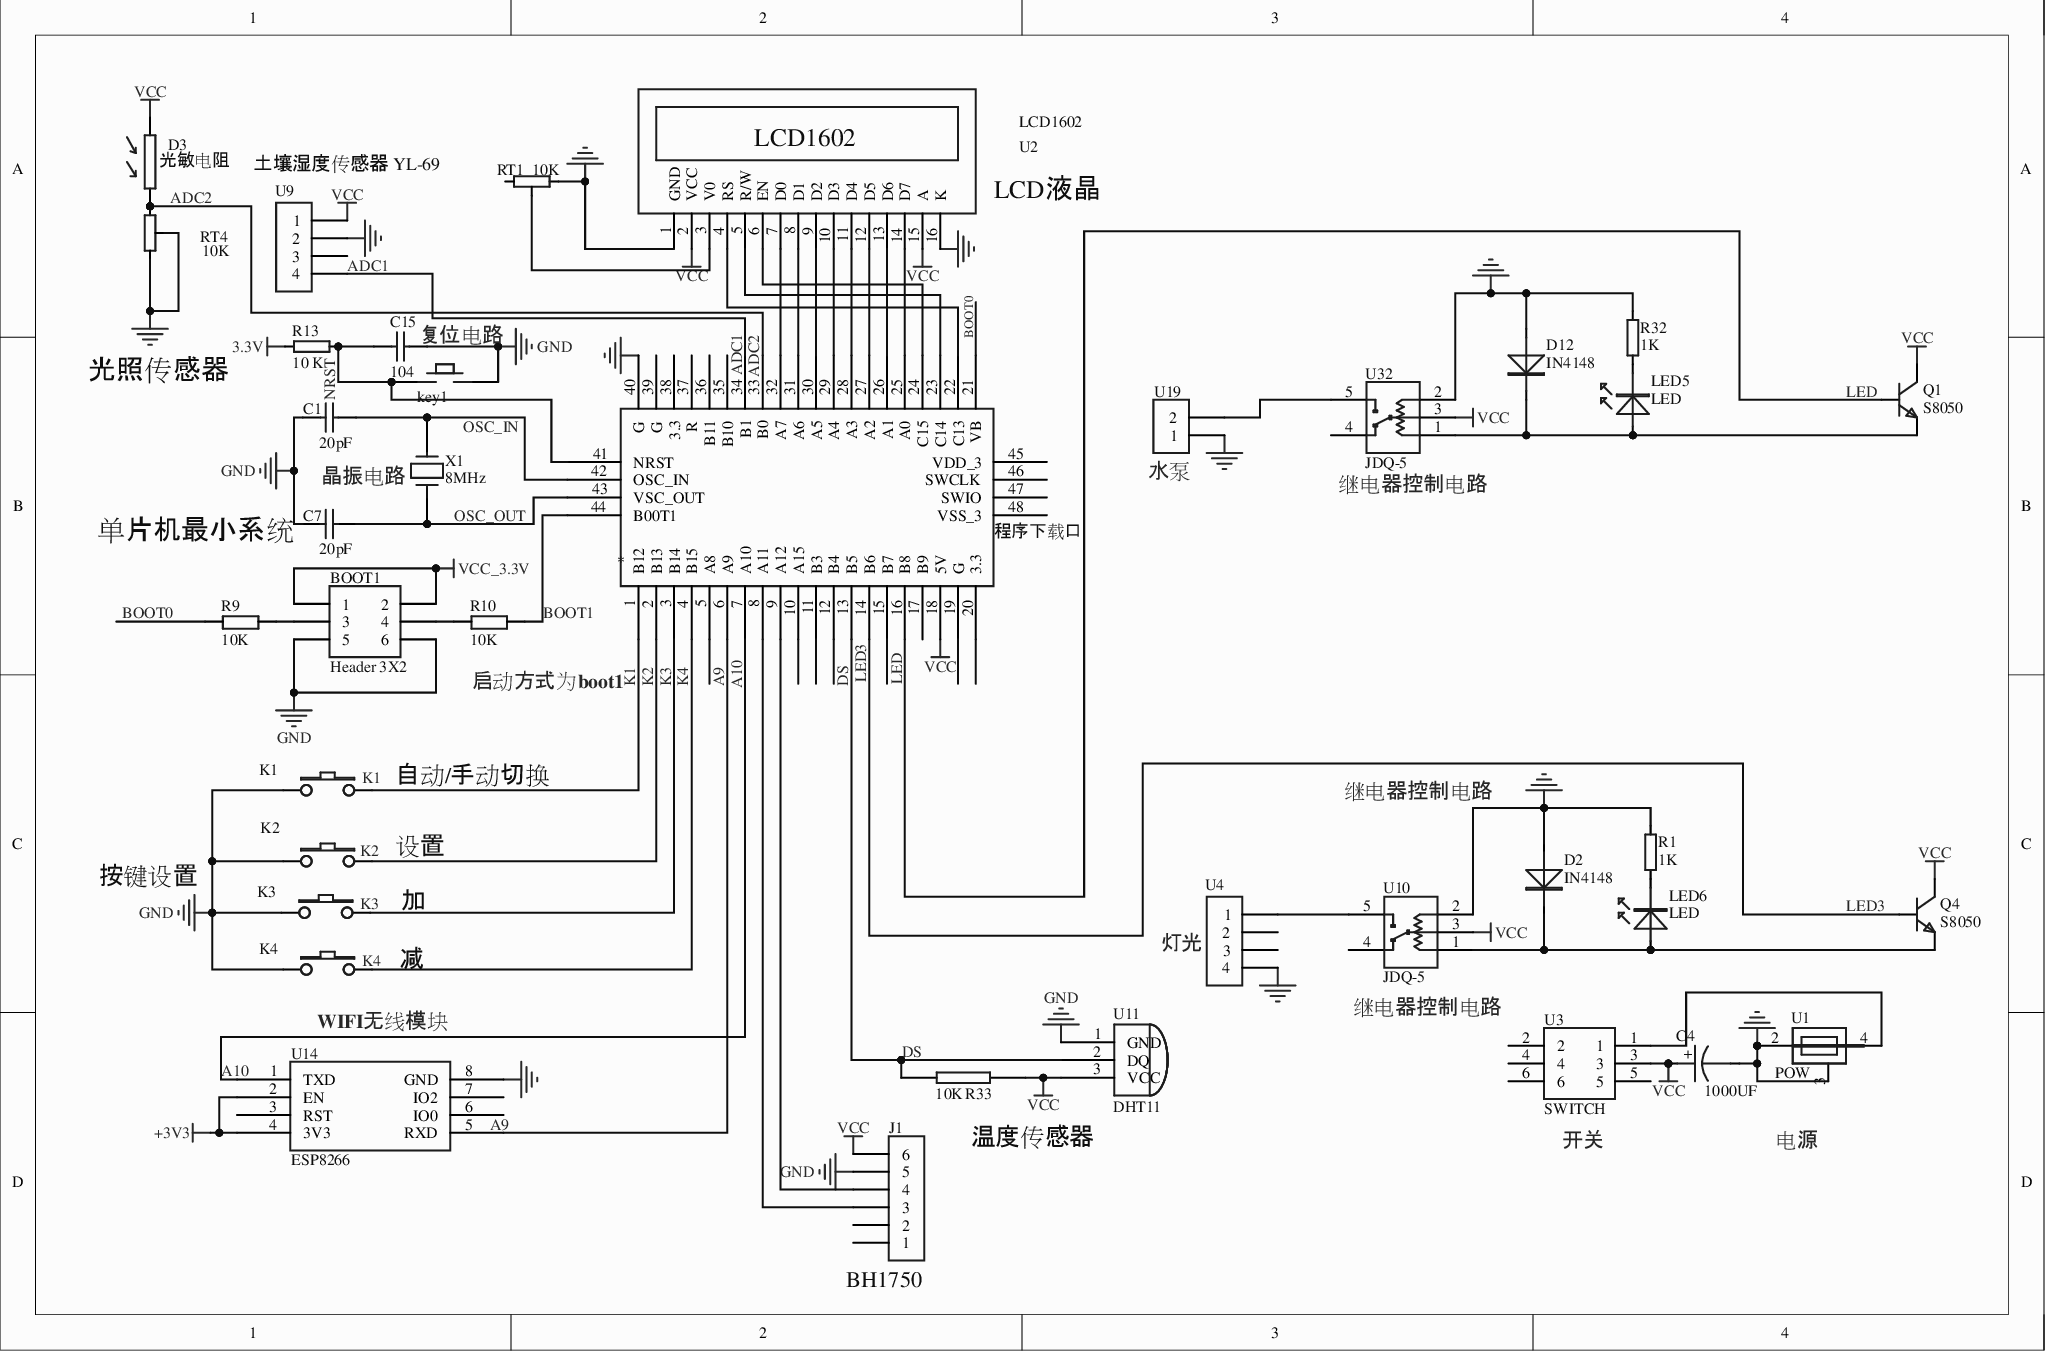
[diagram p0: MISC51945-3.schdoc]
# Altium project MISC51945-2.PrjPcb
1 sheet, 38 parts. Net scope: global (net labels, ports and power ports of the same name join across sheets).
Board file: MISC51945.pcbdoc

## Sheet MISC51945-3.schdoc
size 292 x 193 mm; Name: MISC51945

### Parts
*  程序下载口  [LQFP-48_L7.0-W7.0-P0.50-LS9.0-BL]
BOOT1  Header 3X2  [HDR-TH_6P-P2.54-V-F-R2-C3-S2.54]
C1  20pF  [C0603]
C4  1000UF  [CAP-TH_BD8.0-P3.50-D0.6-FD_1]
C7  20pF  [C0603]
C15  104  [C0603]
D2  IN4148  [SOD-323_L1.8-W1.3-LS2.5-RD]
D3  光敏电阻  [RES-TH_L8.0-W4.4-P4.50-D0.6-S2.0]
D12  IN4148  [SOD-323_L1.8-W1.3-LS2.5-RD]
J1  (no value)  [HDR-TH_6P-P2.54-V-F]
K1  (no value)  [Key_SMD_3x4x2]
K2  (no value)  [Key_SMD_3x4x2]
K3  (no value)  [Key_SMD_3x4x2]
K4  (no value)  [Key_SMD_3x4x2]
key1  KEY_M  [Key_SMD_3x4x2]  (value not drawn)
LED5  LED  [LED0603]
LED6  LED  [LED0603]
Q1  S8050  [S8050_SOT-23]
Q4  S8050  [S8050_SOT-23]
R1  1K  [R0603]
R9  10K  [R0603]
R10  10K  [R0603]
R13  10 K  [R0603]
R32  1K  [R0603]
R33  10K  [R0603]
RT1  10K  [R_3296]
RT4  10K  [R_3296]
U1  POW  [DC-2.0]
U2  LCD1602  [LCD1602]
U3  SWITCH  [SW-TH_6P-L5.8-W5.8-P2.00-LS4.5-TR]
U4  (no value)  [HDR-TH_4P-P2.54-V-F]
U9  (no value)  [HDR-TH_4P-P2.54-V-F]
U10  JDQ-5  [RELAY-TH_FTR-K1CK024W]
U11  DHT11  [HDR-TH_3P-P2.54-V-F]
U14  ESP8266  [WIFIM-TH_8P-L24.7-W14.4-P2.54]
U19  (no value)  [CONN-TH_XH2.54-2P]
U32  JDQ-5  [RELAY-TH_FTR-K1CK024W]
X1  8MHz  [CRYSTAL-SMD_L3.2-W2.5_3225-8MHZ]

### Nets
3.3V: R13.1
+3V3: U14.2(EN) U14.4(3V3)
GND: *.40(G) BOOT1.5 BOOT1.6 C1.1 C4.2 C7.1 C15.1 D2.1(A) D12.1(A) J1.5 K1.1 K2.1 K3.1 K4.1 key1.2 R1.1 R32.1 RT1.3 RT4.1 RT4.2 U1.2 U1.3 U2.1(GND) U2.16(K) U4.4 U9.2 U10.2 U11.1(GND) U14.8(GND) U19.1 U32.2
VCC: *.18(5V) C4.1 D3.1 J1.6 Q1.3(C) Q4.3(C) R33.2 U2.2(VCC) U2.15(A) U3.3 U9.1 U10.3(IN) U11.3(VCC) U32.3(IN)
VCC_3.3V: BOOT1.1 BOOT1.2
A9: *.6(A9) U14.5(RXD)
A10: *.7(A10) U14.1(TXD)
ADC1: *.34(B1) U9.4
ADC2: *.33(B0) D3.2 RT4.3
BOOT0: *.21(VB) R9.1
BOOT1: *.44(B00T1) R10.2
DS: *.13(B5) R33.1 U11.2(DQ)
K1: *.1(B12) K1.2
K2: *.2(B13) K2.2
K3: *.3(B14) K3.2
K4: *.4(B15) K4.2
LED: *.16(B8) Q1.1(B)
LED3: *.14(B6) Q4.1(B)
OSC_OUT: *.43(VSC_OUT) C7.2 X1.1
Net*_8: *.8(A11) J1.3
Net*_9: *.9(A12) J1.4
Net*_22: *.22(C13) U2.4(RS)
Net*_23: *.23(C14) U2.5(R/W)
Net*_24: *.24(C15) U2.6(EN)
Net*_25: *.25(A0) U2.14(D7)
Net*_26: *.26(A1) U2.13(D6)
Net*_27: *.27(A2) U2.12(D5)
Net*_28: *.28(A3) U2.11(D4)
Net*_29: *.29(A4) U2.10(D3)
Net*_30: *.30(A5) U2.9(D2)
Net*_31: *.31(A6) U2.8(D1)
Net*_32: *.32(A7) U2.7(D0)
Net*_41: *.41(NRST) C15.2 key1.1 R13.2
Net*_42: *.42(OSC_IN) C1.2 X1.2
NetBOOT1_3: BOOT1.3 R9.2
NetBOOT1_4: BOOT1.4 R10.1
NetD2_2: D2.2(K) LED6.1 Q4.2(E) U10.1
NetD12_2: D12.2(K) LED5.1 Q1.2(E) U32.1
NetLED5_2: LED5.2 R32.2
NetLED6_2: LED6.2 R1.2
NetRT1_2: RT1.2 U2.3(V0)
NetU1_4: U1.4 U3.1
NetU4_1: U4.1 U10.5(IN)
NetU19_2: U19.2 U32.5(IN)

Not connected (* = marked no-connect by the designer): * 5(A8) 10(A15) 11(B3) 12(B4) 15(B7) 17(B9) 19(G) 20(3.3) 35(B10) 36(B11) 37(R) 38(3.3) 39(G) 45(VDD_3) 46(SWCLK) 47(SWIO) 48(VSS_3); J1 1 2; RT1 1; U3 2 4 5 6; U4 2 3; U9 3; U10 4(IN); U14 3(RST) 6(IO0) 7(IO2); U32 4(IN)

### Notes on the sheet
- (near U9) 土壤湿度传感器 YL-69
- (near U2) LCD液晶
- 光照传感器
- 单片机最小系统
- (near K1) 自动/手动切换
- 设置
- 按键设置
- 加
- 减
- (near R33) 温度传感器
- (near J1) BH1750
- Labels drawn without touching a wire or pin: A9, ADC1, ADC2, K1, K2, K3, K4, NRST, OSC_IN, WIFI无线模块, 启动方式为boot1, 复位电路, 开关, 晶振电路, 水泵, 灯光, 电源, 继电器控制电路

### Library data of the parts
* = 程序下载口: UniqueId: dc55b09e814ab7ff; SymbolName: STM32F103C8T6-2; AddInBom: yes; Device: 程序下载口; DesignItemID: STM32F103C8T6-2; LibraryName: *
BOOT1 = Header 3X2: Header, 3-Pin, Dual row; Origin Footprint: 排针2X3; UniqueId: e60d56c60db38727; AddInBom: yes; Device: Header 3X2; LatestRevisionDate: 17-Jul-2002; LatestRevisionNote: Re-released for DXP Platform.; DesignItemID: Header 3X2; LibraryName: Explorer STM32F407封装库; SymbolName: Header 3X2; Publisher: Altium Limited
C1 = 20pF: Capacitor; Value: 10nF; Origin Footprint: 0603C; UniqueId: 5fb4f22ffcb6a001; SymbolName: Cap; AddInBom: yes; Device: 20pF; Published: 8-Jun-2000; Revision: July-2002: Re-released for DXP Platform.; DesignItemID: Cap; LibraryName: MyLib; Publisher: Altium Limited
C4 = 1000UF: Origin Footprint: C10; UniqueId: 623e2bb2442f04df; SymbolName: 10uF; AddInBom: yes; Device: 1000UF; DesignItemID: 10uF; LibraryName: *
C7 = 20pF: Capacitor; Value: 10nF; Origin Footprint: 0603C; UniqueId: 3007ca2539a35480; SymbolName: Cap; AddInBom: yes; Device: 20pF; Published: 8-Jun-2000; Revision: July-2002: Re-released for DXP Platform.; DesignItemID: Cap; LibraryName: MyLib; Publisher: Altium Limited
C15 = 104: Capacitor; Value: 10nF; Origin Footprint: 0603C; UniqueId: 4a0fa0f8d5a09ecc; SymbolName: Cap; AddInBom: yes; Device: 104; Published: 8-Jun-2000; Revision: July-2002: Re-released for DXP Platform.; DesignItemID: Cap; LibraryName: MyLib; Publisher: Altium Limited
D2 = IN4148: UniqueId: fa5cd661465da5bc; SymbolName: DIODE; AddInBom: yes; Device: IN4148; Origin Footprint: IN4148; DesignItemID: DIODE; LibraryName: *
D3 = 光敏电阻: Origin Footprint: SIP2; UniqueId: ce0e29427420bb9a; SymbolName: RES4; AddInBom: yes; Device: 光敏电阻; DesignItemID: RES4; LibraryName: *
D12 = IN4148: UniqueId: b8e2e60fde6cbaf9; SymbolName: DIODE; AddInBom: yes; Device: IN4148; Origin Footprint: IN4148; DesignItemID: DIODE; LibraryName: *
J1 = J?: Origin Footprint: Fe-HDR1X6/2.54-S; UniqueId: f1a4251ed188e02c; SymbolName: Female HDR1X6; AddInBom: yes; Device: J?; DesignItemID: Female HDR1X6; LibraryName: 排母
K1 = K1: Origin Footprint: KEY1; UniqueId: 28855386baaab8ba; AddInBom: yes; ModelId: c49c161387de499d88b938ca9a66f7e2; Device: K1; DesignItemID: KEY1; LibraryName: 51SCH; SymbolName: KEY1; ModelName: KEY1
K2 = K2: Origin Footprint: KEY1; UniqueId: e2dee5ee6a5fdee0; AddInBom: yes; ModelId: c49c161387de499d88b938ca9a66f7e2; Device: K2; DesignItemID: KEY1; LibraryName: 51SCH; SymbolName: KEY1; ModelName: KEY1
K3 = K3: Origin Footprint: KEY1; UniqueId: 177bbada0502c5f7; AddInBom: yes; ModelId: c49c161387de499d88b938ca9a66f7e2; Device: K3; DesignItemID: KEY1; LibraryName: 51SCH; SymbolName: KEY1; ModelName: KEY1
K4 = K4: Origin Footprint: KEY1; UniqueId: 787baf109c0c5026; AddInBom: yes; ModelId: c49c161387de499d88b938ca9a66f7e2; Device: K4; DesignItemID: KEY1; LibraryName: 51SCH; SymbolName: KEY1; ModelName: KEY1
key1 = KEY_M: Origin Footprint: 按键; UniqueId: ee3cfa7ccfc084a0; AddInBom: yes; Device: KEY_M; DesignItemID: KEY_M; LibraryName: mylib; SymbolName: KEY_M
LED5 = LED: UniqueId: 1218a8b603bcfedf; AddInBom: yes; Device: LED; Origin Footprint: LED; DesignItemID: LED; LibraryName: *; SymbolName: LED
LED6 = LED: UniqueId: 1801f051ed571ab9; AddInBom: yes; Device: LED; Origin Footprint: LED; DesignItemID: LED; LibraryName: *; SymbolName: LED
Q1 = S8050: Origin Footprint: PNP; UniqueId: 047b734180970fea; SymbolName: NPN; AddInBom: yes; Device: S8050; DesignItemID: NPN; LibraryName: *
Q4 = S8050: Origin Footprint: PNP; UniqueId: 3881765f76976367; SymbolName: NPN; AddInBom: yes; Device: S8050; DesignItemID: NPN; LibraryName: *
R1 = 1K: Origin Footprint: R-DIP; UniqueId: gge2; AddInBom: yes; Device: 1K; DesignItemID: 1K; LibraryName: *; SymbolName: 1K
R9 = 10K_1: Origin Footprint: 0603R; UniqueId: 7a9d276dcc23a651; SymbolName: R; AddInBom: yes; Device: 10K_1; DesignItemID: R; LibraryName: Explorer STM32F407封装库
R10 = 10K_1: Origin Footprint: 0603R; UniqueId: 7663007c1f2bc029; SymbolName: R; AddInBom: yes; Device: 10K_1; DesignItemID: R; LibraryName: Explorer STM32F407封装库
R13 = 10 K: Origin Footprint: R-DIP; UniqueId: ff7631ddbc1e2fda; SymbolName: 1K; AddInBom: yes; Device: 10 K; DesignItemID: 1K; LibraryName: 51SCH
R32 = 1K: Origin Footprint: R-DIP; UniqueId: 0b1dfdee8a75b846; AddInBom: yes; Device: 1K; DesignItemID: 1K; LibraryName: *; SymbolName: 1K
R33 = 10K_2: Origin Footprint: R-DIP; UniqueId: c45f10131c8227f7; SymbolName: RES2; AddInBom: yes; Device: 10K_2; DesignItemID: RES2; LibraryName: *
RT1 = 10K: Origin Footprint: RT1; UniqueId: 0e537e034f78096e; SymbolName: RT; AddInBom: yes; Device: 10K; DesignItemID: RT; LibraryName: *
RT4 = 10K: Origin Footprint: RT1; UniqueId: 35b8b4d1d992c2bc; SymbolName: RT; AddInBom: yes; Device: 10K; DesignItemID: RT; LibraryName: *
U1 = POW: Origin Footprint: DCM; Symbol: POW_1; UniqueId: gge1; AddInBom: yes; Device: POW; DesignItemID: POW; LibraryName: *
U2 = LCD1602: UniqueId: d74c11912b695046; AddInBom: yes; ModelId: f9d832f46a914cadb50fc4d4cefd2517; Device: LCD1602; DesignItemID: LCD1602; LibraryName: *; SymbolName: LCD1602; FootprintName: LCD1602; ModelName: LCD1602
U3 = SWITCH: Origin Footprint: KG1; UniqueId: eac3f191c372887e; AddInBom: yes; Device: SWITCH; DesignItemID: SWITCH; LibraryName: *; SymbolName: SWITCH
U4 = U9: Connector; Origin Footprint: SIP4; UniqueId: gge3; SymbolName: CON4; AddInBom: yes; Device: U9; DesignItemID: CON4; LibraryName: *
U9 = U9: Connector; Origin Footprint: SIP4; UniqueId: 0cf0c6d72374702e; SymbolName: CON4; AddInBom: yes; Device: U9; DesignItemID: CON4; LibraryName: *
U10 = JDQ-5: UniqueId: 5152fb4fa8412479; AddInBom: yes; Device: JDQ-5; Origin Footprint: JDQ-5; DesignItemID: JDQ-5; LibraryName: *; SymbolName: JDQ-5
U11 = DHT11: Origin Footprint: SIP3; UniqueId: 8cd974130b34484c; SymbolName: DS18B20; AddInBom: yes; Device: DHT11; DesignItemID: DS18B20; LibraryName: *
U14 = ESP8266: Origin Footprint: SIP-4-2-H; UniqueId: 02f5647e0f4b6551; SymbolName: Component_2; AddInBom: yes; Device: ESP8266; DesignItemID: Component_2; LibraryName: *
U19 = U19: Origin Footprint: SIP2; UniqueId: 8620e459a4cf64b8; SymbolName: CON2; AddInBom: yes; Device: U19; DesignItemID: CON2; LibraryName: *
U32 = JDQ-5: UniqueId: 52dbb124fa963d8c; AddInBom: yes; Device: JDQ-5; Origin Footprint: JDQ-5; DesignItemID: JDQ-5; LibraryName: *; SymbolName: JDQ-5
X1 = 8MHz: Crystal; Origin Footprint: 晶振8M; UniqueId: 3fdc0bfeb28a4101; AddInBom: yes; Device: 8MHz; DesignItemID: CRYSTAL; LibraryName: MyLib; SymbolName: CRYSTAL